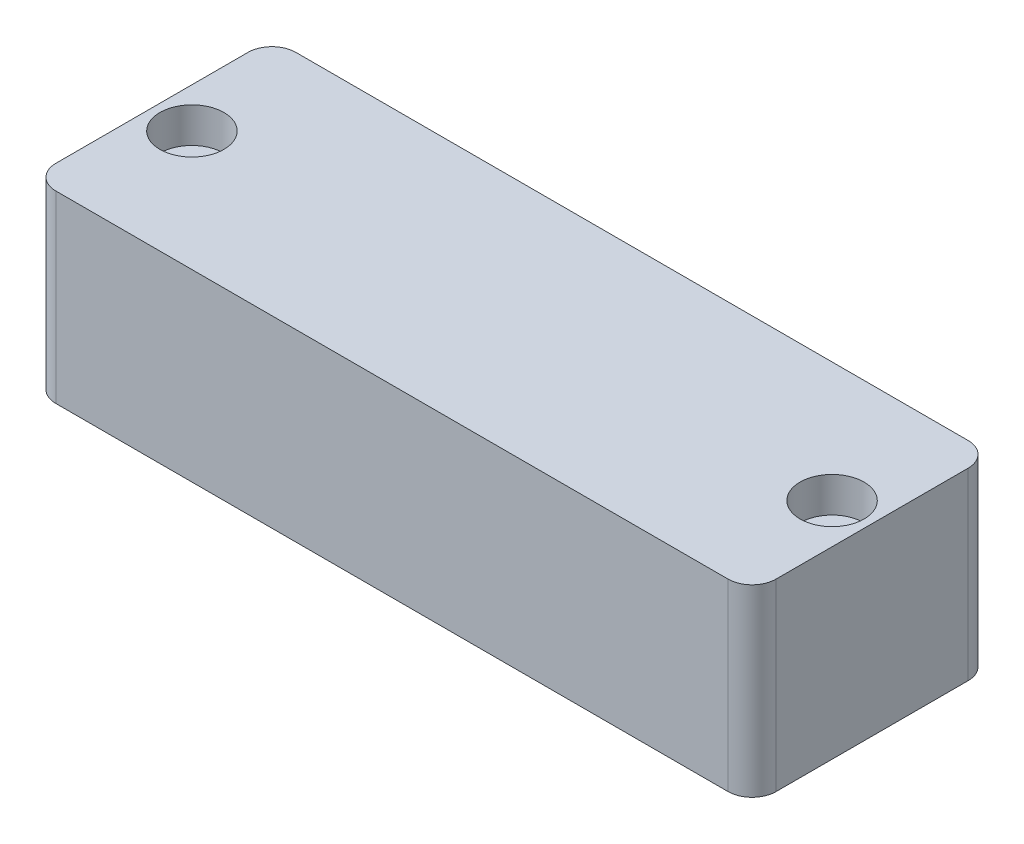
SolidWorks part; units mm, degrees
material "标准件"
ref_plane "前视基准面" through (0, 0, 0) normal (0, 0, 1) x (1, 0, 0)
ref_plane "上视基准面" through (0, 0, 0) normal (0, 1, 0) x (1, 0, 0)
ref_plane "右视基准面" through (0, 0, 0) normal (1, 0, 0) x (0, 0, -1)
sketch "草图1" plane through (0, 0, 0) normal (0, 1, 0) x (1, 0, 0)
  line L1 (-45, -15) -> (45, -15)
  line L2 (-45, -15) -> (-45, 15)
  line L3 (-45, 15) -> (45, 15)
  line L4 (45, -15) -> (45, 15)
  line L5 (-45, -15) -> (45, 15) construction
  line L6 (-45, 15) -> (45, -15) construction
  point P0 (0, 0)
  dimension "D1" = 90
  dimension "D2" = 30
extrude "凸台-拉伸1" add sketch "草图1" along normal mid plane 23
hole_wizard "M4 六角凹头螺钉的柱形沉头孔1" positions "草图2" profile "草图3" counterbore size "M4" standard "ISO" end condition through all
sketch "草图2" plane through (0, 11.5, 0) normal (0, 1, 0) x (1, 0, 0)
  line L0 (0, 0) -> (0, 32.2434) construction
  point P0 (-40, 0)
  point P2 (40, 0)
  dimension "D1" = 80
sketch "草图3" plane through (-40, 11.5, 0) normal (1, 0, 0) x (0, 0, 1)
  line L0 (0, 0) -> (0, 23)
  line L1 (0, 23) -> (2.25, 23)
  line L3 (2.25, 23) -> (2.25, 4.4)
  line L4 (2.25, 4.4) -> (4, 4.4)
  line L5 (4, 4.4) -> (4, 0)
  line L7 (4, 0) -> (0, 0)
  line L11 (0, -6.35) -> (0, 107.95) construction
  dimension "通孔孔直径" = 4.5
  dimension "通孔孔深度" = 23
  dimension "柱形沉头孔直径" = 8
  dimension "柱形沉头孔深度" = 4.4
fillet "圆角1" radius 3 4 edges at (45, 0, 15) (45, 0, -15) (-45, 0, -15) (-45, 0, 15)
